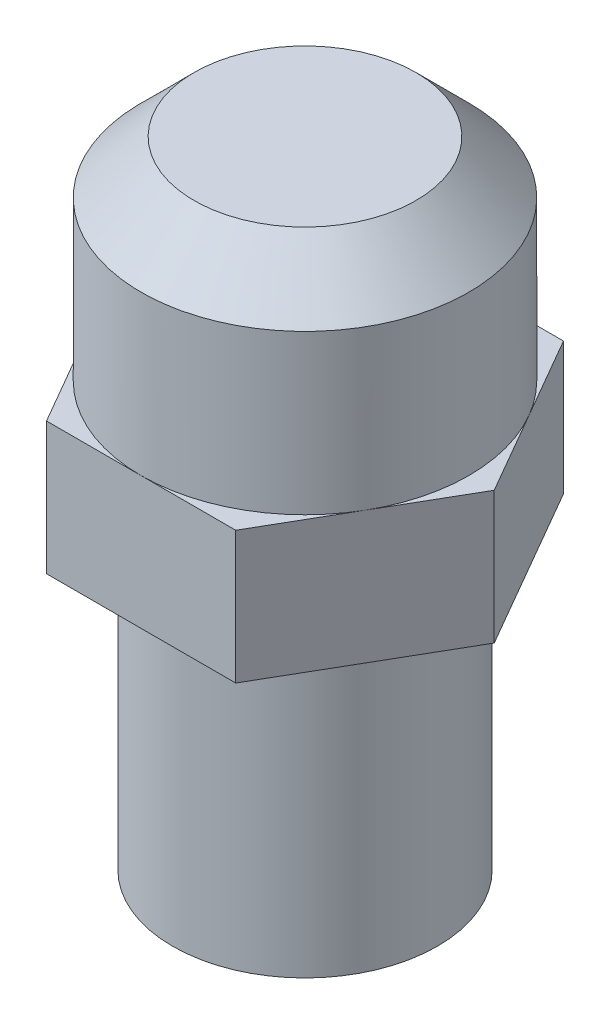
SolidWorks part; units mm, degrees
material "PP 共聚物"
ref_plane "前视基准面" through (0, 0, 0) normal (0, 0, 1) x (1, 0, 0)
ref_plane "上视基准面" through (0, 0, 0) normal (0, 1, 0) x (1, 0, 0)
ref_plane "右视基准面" through (0, 0, 0) normal (1, 0, 0) x (0, 0, -1)
sketch "草图1" plane through (0, 0, 0) normal (0, 1, 0) x (1, 0, 0)
  line L1 (-7.15, 0) -> (-3.575, -6.1921)
  line L2 (-3.575, -6.1921) -> (3.575, -6.1921)
  line L3 (3.575, -6.1921) -> (7.15, 0)
  line L4 (7.15, 0) -> (3.575, 6.1921)
  line L5 (3.575, 6.1921) -> (-3.575, 6.1921)
  line L6 (-3.575, 6.1921) -> (-7.15, 0)
  circle A0 centre (0, 0) radius 6.1921 construction
  dimension "D1" = 14.3
extrude "凸台-拉伸1" add sketch "草图1" along normal blind 5
sketch "草图2" plane through (0, 5, 0) normal (0, 1, 0) x (1, 0, 0)
  line L0 (3.575, 6.1921) -> (-3.575, 6.1921) construction
  circle A0 centre (0, 0) radius 6.1921
extrude "凸台-拉伸2" add sketch "草图2" along normal blind 8
chamfer "倒角1" distance 2 angle 45 1 edges at (0, 13, 6.1921)
sketch "草图3" plane through (0, 0, 0) normal (0, -1, 0) x (1, 0, 0)
  circle A0 centre (0, 0) radius 5
  dimension "D1" = 10
extrude "凸台-拉伸3" add sketch "草图3" along normal blind 11
